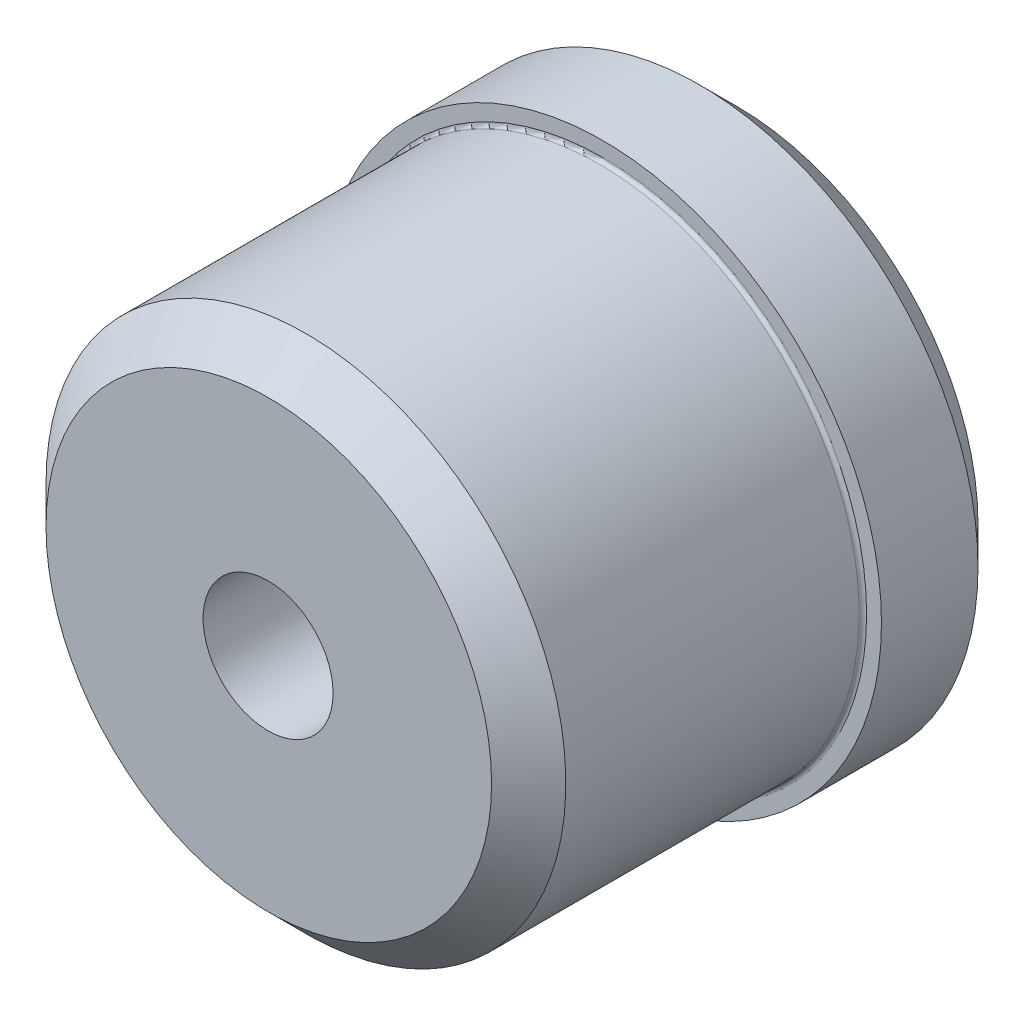
SolidWorks part; units mm, degrees
material "42CrMo"
ref_plane "前视基准面" through (0, 0, 0) normal (0, 0, 1) x (1, 0, 0)
ref_plane "上视基准面" through (0, 0, 0) normal (0, 1, 0) x (1, 0, 0)
ref_plane "右视基准面" through (0, 0, 0) normal (1, 0, 0) x (0, 0, -1)
sketch "草图1" plane through (0, 0, 0) normal (0, 0, 1) x (1, 0, 0)
  circle A0 centre (0, 0) radius 35
  dimension "D1" = 70
extrude "凸台-拉伸1" add sketch "草图1" along normal blind 45
sketch "草图5" plane through (0, 0, 0) normal (0, 0, -1) x (-1, 0, 0)
  circle A0 centre (0, 0) radius 37.5
  dimension "D1" = 75
extrude "凸台-拉伸2" add sketch "草图5" along normal blind 18
chamfer "倒角1" distance 5 angle 45 2 edges at (35, 0, 45) (-37.5, 0, -18)
hole_wizard "M20 螺纹孔1" positions "3D草图2" profile "草图4" tap size "M20" standard "GB" end condition through all
sketch3d "3D草图2"
  point P0 (-0.0934, -0.1401, 45)
cosmetic thread "孔螺蚊线1" parameters "D2"=20
sketch "草图4" plane through (-0.0934, -0.1401, 45) normal (1, 0, 0) x (0, -1, 0)
  line L0 (0, 0) -> (0, 63)
  line L1 (0, 63) -> (8.75, 63)
  line L2 (8.75, 63) -> (8.75, 0)
  line L5 (8.75, 0) -> (0, 0)
  line L11 (0, -6.35) -> (0, 107.95) construction
  dimension "通孔螺纹孔钻头直径" = 17.5
  dimension "通孔螺纹孔钻头深度" = 63
fillet "圆角1" radius 0.5 1 edges at (35, 0, 0)
